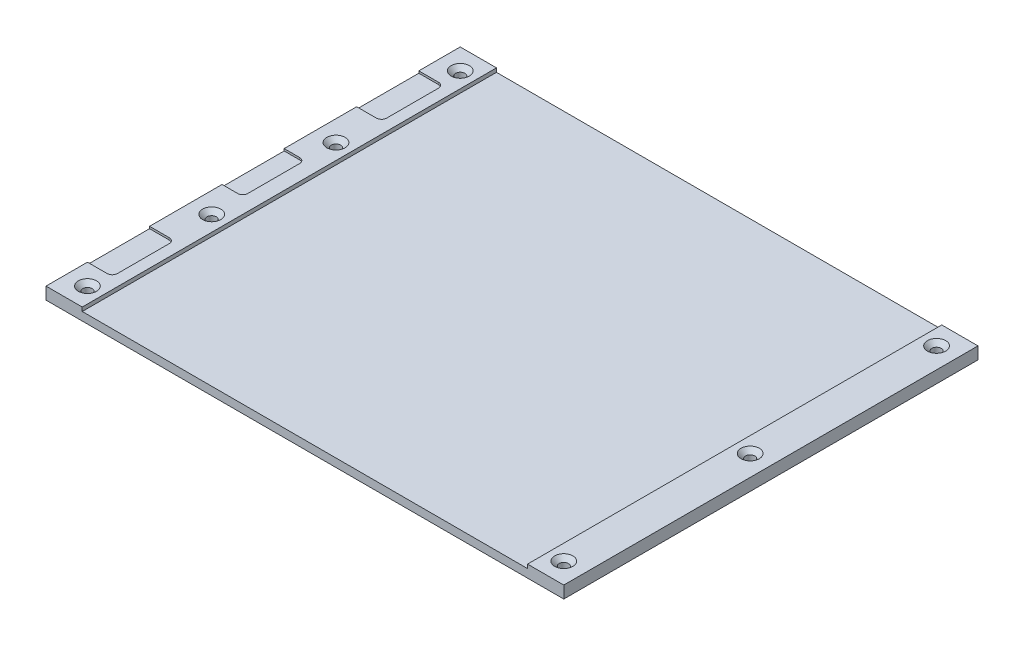
from build123d import *

# Parameters (mm, degrees)
SKETCH1_W                                           = 500
SKETCH1_H                                           = 24
BOSS_EXTRUDE1_DEPTH                                 = 400
SKETCH2_W                                           = 430
SKETCH2_H                                           = 8
CUT_EXTRUDE1_DEPTH                                  = 641.762046317
SKETCH3_W                                           = 544.957019416
SKETCH3_H                                           = 0.5
CUT_EXTRUDE2_DEPTH                                  = 641.762046317
SKETCH12_W                                          = 569.007892772
SKETCH12_H                                          = 39.328779912
CUT_EXTRUDE3_DEPTH                                  = 641.762046317
HOLE_WIZARD_HEX_SOCKET_SEMI_COUNTERSUNK_D           = 9
HOLE_WIZARD_HEX_SOCKET_SEMI_COUNTERSUNK_CSINK_D     = 17.6
HOLE_WIZARD_HEX_SOCKET_SEMI_COUNTERSUNK_CSINK_ANGLE = 90
SKETCH16_W                                          = 24
SKETCH16_H                                          = 60
SKETCH16_W_2                                        = 20
CUT_EXTRUDE4_DEPTH                                  = 2
FILLET1_R                                           = 5
HOLE_WIZARD_HEX_SOCKET_SEMI_COUNTER_2_D             = 9
HOLE_WIZARD_HEX_SOCKET_SEMI_COUNTER_2_CSINK_D       = 17.6
HOLE_WIZARD_HEX_SOCKET_SEMI_COUNTER_2_CSINK_ANGLE   = 90


with BuildPart() as part:
    # Sketch1 → Boss-Extrude1 (new body)
    with BuildSketch(Plane.XY):
        with Locations((250, 12)):
            Rectangle(SKETCH1_W, SKETCH1_H)
    extrude(amount=-BOSS_EXTRUDE1_DEPTH)

    # Sketch2 → Cut-Extrude1 (cut, through all)
    with BuildSketch(Plane.XY):
        with Locations((250, 12)):
            Rectangle(SKETCH2_W, SKETCH2_H)
    extrude(amount=-CUT_EXTRUDE1_DEPTH, mode=Mode.SUBTRACT)

    # Sketch3 → Cut-Extrude2 (cut, through all)
    with BuildSketch(Plane.XY):
        with Locations((250, 12)):
            Rectangle(SKETCH3_W, SKETCH3_H)
    extrude(amount=-CUT_EXTRUDE2_DEPTH, mode=Mode.SUBTRACT)


with BuildPart() as cut_extrude2_piece_1:
    # of the separate pieces the step leaves, piece 1, a body of its own (cut_extrude2_pieces)
    add(part.part.solids().sort_by_distance((0, 0, 0))[0])

    # Hole wizard_ hex socket semi-countersunk (through all)
    with Locations(Plane(origin=(0, 11.75, 0), x_dir=(1, 0, 0), z_dir=(0, 1, 0))):
        with Locations((20, 20), (480, 20), (20, 380), (480, 380)):
            CounterSinkHole(HOLE_WIZARD_HEX_SOCKET_SEMI_COUNTERSUNK_D / 2, HOLE_WIZARD_HEX_SOCKET_SEMI_COUNTERSUNK_CSINK_D / 2, counter_sink_angle=HOLE_WIZARD_HEX_SOCKET_SEMI_COUNTERSUNK_CSINK_ANGLE)

    # Sketch16 → Cut-Extrude4 (cut)
    with BuildSketch(Plane(origin=(0, 11.75, 0), x_dir=(1, 0, 0), z_dir=(0, 1, 0))):
        with Locations((12, 330)):
            Rectangle(SKETCH16_W, SKETCH16_H)
        with Locations((12, 70)):
            Rectangle(SKETCH16_W, SKETCH16_H)
        with Locations((10, 200)):
            Rectangle(SKETCH16_W_2, SKETCH16_H)
    extrude(amount=-CUT_EXTRUDE4_DEPTH, mode=Mode.SUBTRACT)

    # Fillet1
    fillet1_edges = [cut_extrude2_piece_1.edges().sort_by_distance(p)[0] for p in [
        (24, 10.75, -360),
        (24, 10.75, -300),
        (24, 10.75, -40),
        (24, 10.75, -100),
        (20, 10.75, -230),
        (20, 10.75, -170),
    ]]
    fillet(fillet1_edges, radius=FILLET1_R)

    # Hole wizard_ hex socket semi-counter 2 (through all)
    with Locations(Plane(origin=(0, 11.75, 0), x_dir=(1, 0, 0), z_dir=(0, 1, 0))):
        with Locations((20, 140), (20, 260), (480, 200)):
            CounterSinkHole(HOLE_WIZARD_HEX_SOCKET_SEMI_COUNTER_2_D / 2, HOLE_WIZARD_HEX_SOCKET_SEMI_COUNTER_2_CSINK_D / 2, counter_sink_angle=HOLE_WIZARD_HEX_SOCKET_SEMI_COUNTER_2_CSINK_ANGLE)


with BuildPart() as cut_extrude2_piece_2:
    # of the separate pieces the step leaves, piece 2, a body of its own (cut_extrude2_pieces)
    add(part.part.solids().sort_by_distance((0, 24, 0))[0])

    # Sketch12 → Cut-Extrude3 (cut, through all)
    with BuildSketch(Plane.XY):
        with Locations((265.175540793, 31.664389956)):
            Rectangle(SKETCH12_W, SKETCH12_H)
    extrude(amount=-CUT_EXTRUDE3_DEPTH, mode=Mode.SUBTRACT)


solid = cut_extrude2_piece_1.part
